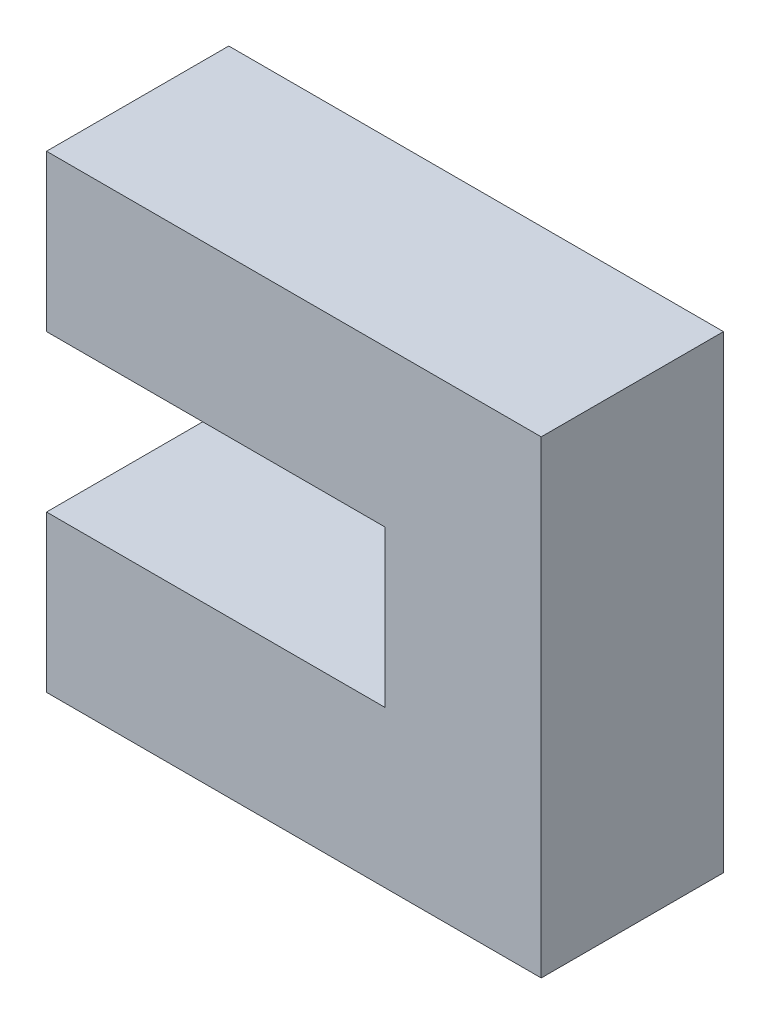
SolidWorks part; units mm, degrees
ref_plane "前视基准面" through (0, 0, 0) normal (0, 0, 1) x (1, 0, 0)
ref_plane "上视基准面" through (0, 0, 0) normal (0, 1, 0) x (1, 0, 0)
ref_plane "右视基准面" through (0, 0, 0) normal (1, 0, 0) x (0, 0, -1)
sketch "草图1" plane through (0, 0, 0) normal (0, 0, 1) x (1, 0, 0)
  line L0 (0, 0) -> (0, 9)
  line L1 (0, 9) -> (-19, 9)
  line L2 (-19, 9) -> (-19, 3)
  line L3 (-19, 3) -> (-6, 3)
  line L4 (-6, 3) -> (-6, -3)
  line L5 (-6, -3) -> (-19, -3)
  line L6 (-19, -3) -> (-19, -9)
  line L7 (-19, -9) -> (0, -9)
  line L8 (0, -9) -> (0, 0)
  dimension "D1" = 6
  dimension "D2" = 6
  dimension "D3" = 6
  dimension "D4" = 13
extrude "凸台-拉伸1" add sketch "草图1" along normal mid plane 7
